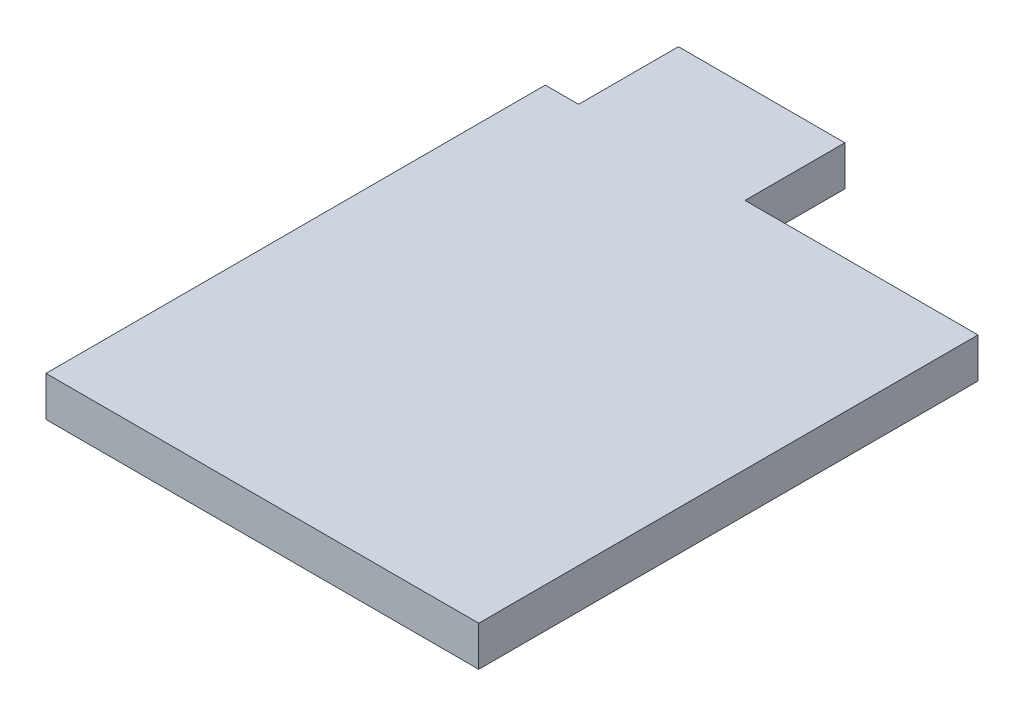
SolidWorks part; units mm, degrees
ref_plane "前视基准面" through (0, 0, 0) normal (0, 0, 1) x (1, 0, 0)
ref_plane "上视基准面" through (0, 0, 0) normal (0, 1, 0) x (1, 0, 0)
ref_plane "右视基准面" through (0, 0, 0) normal (1, 0, 0) x (0, 0, -1)
sketch "草图1" plane through (0, 0, 0) normal (0, 1, 0) x (1, 0, 0)
  line L0 (0, 0) -> (130, 0)
  line L1 (130, 0) -> (130, 150)
  line L2 (130, 150) -> (60, 150)
  line L3 (60, 150) -> (60, 180)
  line L4 (60, 180) -> (10, 180)
  line L5 (10, 180) -> (10, 150)
  line L6 (10, 150) -> (0, 150)
  line L7 (0, 150) -> (0, 0)
  dimension "D1" = 130
  dimension "D2" = 150
  dimension "D3" = 50
  dimension "D4" = 70
  dimension "D5" = 30
extrude "凸台-拉伸1" add sketch "草图1" along normal blind 12
